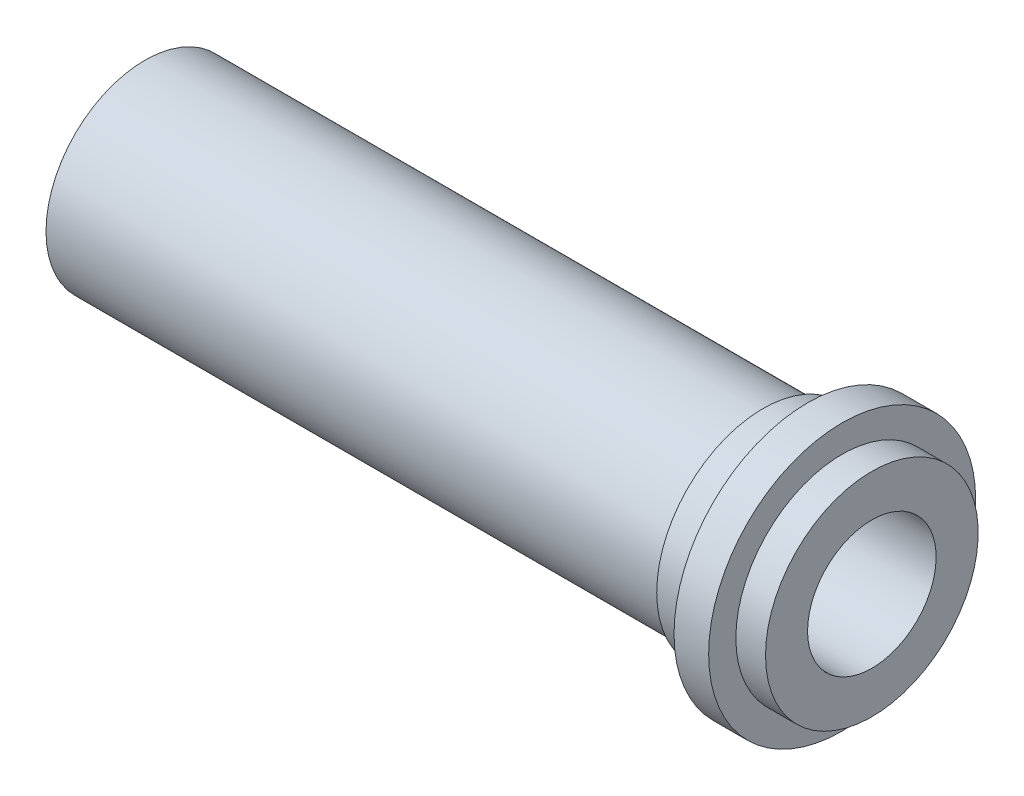
from build123d import *

# Parameters (mm, degrees)
EXTRUDE_START   = -6
SKETCH_2_R      = 27
SKETCH_2_R_2    = 21.5
EXTRUDE_1_DEPTH = 7


with BuildPart() as part:
    # 草图1 → 旋转1 (revolve)
    with BuildSketch(Plane.XY, mode=Mode.PRIVATE) as revolve_1_sk:
        Polygon((0, 13), (0, 20), (125, 20), (125, 21.5), (147, 21.5), (147, 13), align=None)
    revolve(revolve_1_sk.sketch.rotate(Axis((0, 0, 0), (1, 0, 0)), 90), axis=Axis((0, 0, 0), (1, 0, 0)))

    # 草图2 → 凸台-拉伸1 (add)
    with BuildSketch(Plane(origin=(147, 0, 0), x_dir=(0, 0, -1), z_dir=(1, 0, 0)).offset(EXTRUDE_START)):
        Circle(SKETCH_2_R)
        with Locations(Location((0, 0, 0), (0, 0, 180))):
            Circle(SKETCH_2_R_2, mode=Mode.SUBTRACT)
    extrude(amount=-EXTRUDE_1_DEPTH)


solid = part.part
